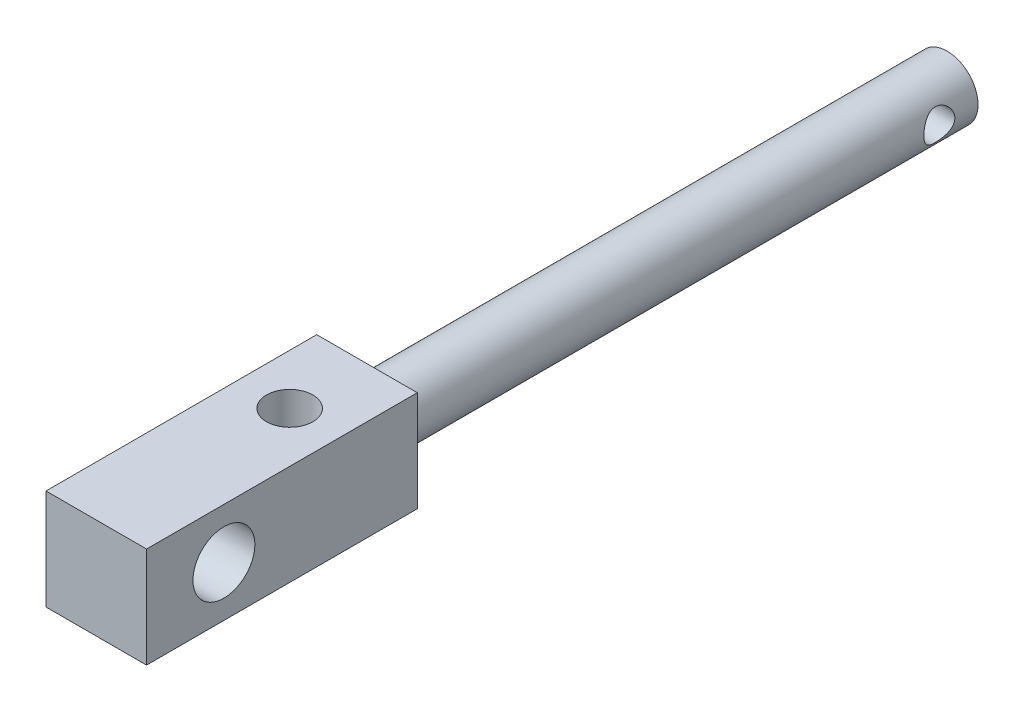
from build123d import *

# Parameters (mm, degrees)
SKETCH_1_W          = 13
SKETCH_1_H          = 13
EXTRUDE_1_DEPTH     = 10
SKETCH_3_R          = 3
CUT_EXTRUDE_1_DEPTH = 20
SKETCH_4_R          = 4
EXTRUDE_2_DEPTH     = 75
SKETCH_5_W          = 13
SKETCH_5_H          = 13
EXTRUDE_3_DEPTH     = 15
SKETCH_6_R          = 4
CUT_EXTRUDE_2_DEPTH = 37
SKETCH_7_R          = 2
CUT_EXTRUDE_3_DEPTH = 300


with BuildPart() as part:
    # 草图1 → 凸台-拉伸1 (new, symmetric)
    with BuildSketch(Plane.XY):
        Rectangle(SKETCH_1_W, SKETCH_1_H)
    extrude(amount=EXTRUDE_1_DEPTH, both=True)

    # 草图3 → 切除-拉伸1 (cut)
    with BuildSketch(Plane(origin=(0, 6.5, 0), x_dir=(1, 0, 0), z_dir=(0, 1, 0))):
        with Locations(Location((0, 0, 0), (0, 0, 180))):
            Circle(SKETCH_3_R)
    extrude(amount=-CUT_EXTRUDE_1_DEPTH, mode=Mode.SUBTRACT)

    # 草图4 → 凸台-拉伸2 (add)
    with BuildSketch(Plane(origin=(0, 0, -10), x_dir=(-1, 0, 0), z_dir=(0, 0, -1))):
        Circle(SKETCH_4_R)
    extrude(amount=EXTRUDE_2_DEPTH)

    # 草图5 → 凸台-拉伸3 (add)
    with BuildSketch(Plane.XY.offset(10)):
        Rectangle(SKETCH_5_W, SKETCH_5_H)
    extrude(amount=EXTRUDE_3_DEPTH)

    # 草图6 → 切除-拉伸2 (cut)
    with BuildSketch(Plane.ZY.offset(6.5)):
        with Locations((15, 0)):
            Circle(SKETCH_6_R)
    extrude(amount=-CUT_EXTRUDE_2_DEPTH, mode=Mode.SUBTRACT)

    # 草图7 → 切除-拉伸3 (cut)
    with BuildSketch(Plane.ZY.offset(6.5)):
        with Locations(Location((-80, 0, 0), (0, 0, 179.999999996))):
            Circle(SKETCH_7_R)
    extrude(amount=-CUT_EXTRUDE_3_DEPTH, mode=Mode.SUBTRACT)


solid = part.part
